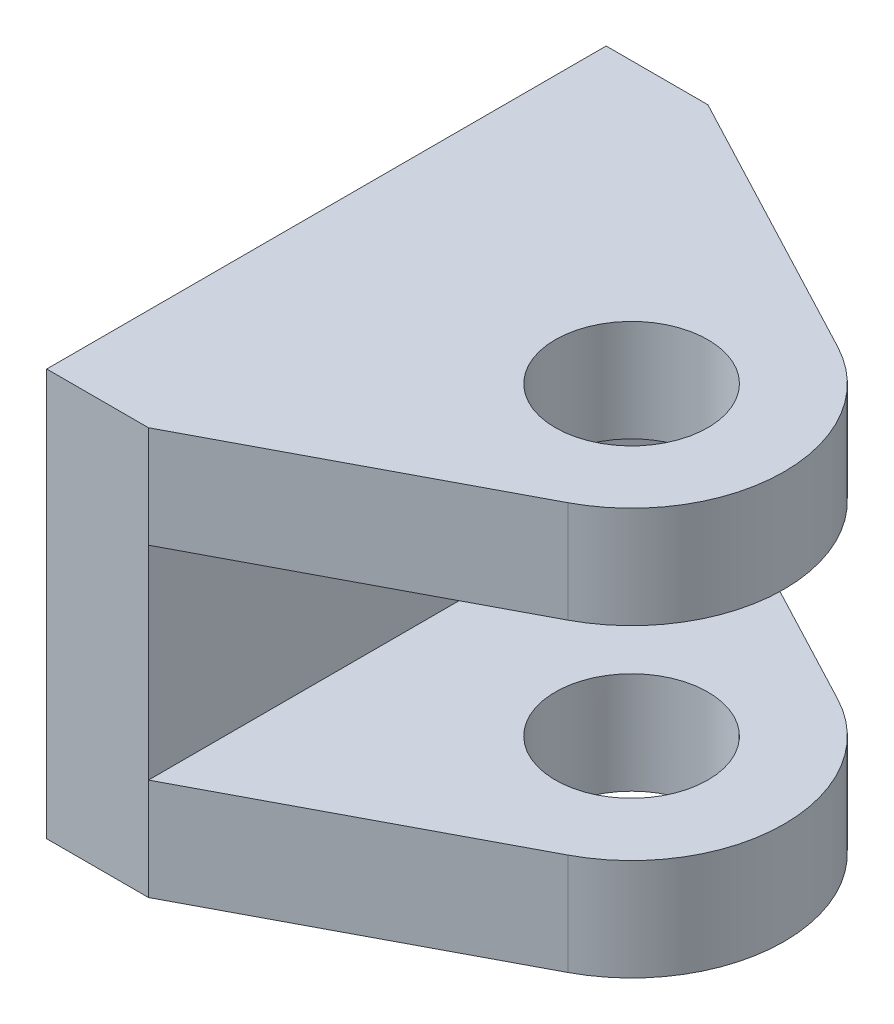
SolidWorks part; units mm, degrees
material "合金钢"
ref_plane "前视基准面" through (0, 0, 0) normal (0, 0, 1) x (1, 0, 0)
ref_plane "上视基准面" through (0, 0, 0) normal (0, 1, 0) x (1, 0, 0)
ref_plane "右视基准面" through (0, 0, 0) normal (1, 0, 0) x (0, 0, -1)
sketch "草图1" plane through (0, 0, 0) normal (0, 1, 0) x (1, 0, 0)
  line L0 (0, -27.5) -> (0, 27.5)
  line L1 (0, -27.5) -> (10, -27.5)
  line L2 (10, -27.5) -> (36.995, -13.2691)
  line L3 (0, 27.5) -> (10, 27.5)
  line L4 (10, 27.5) -> (36.995, 13.2691)
  arc A0 (36.995, -13.2691) -> (36.995, 13.2691) centre (30, 0) ccw
  circle A1 centre (30, 0) radius 7.5
  point P4 (0, 0)
  dimension "D1" = 30
  dimension "D2" = 15
  dimension "D3" = 10
  dimension "D4" = 10
  dimension "D5" = 30
  dimension "D6" = 55
extrude "凸台-拉伸1" add sketch "草图1" along normal blind 40
sketch "草图2" plane through (0, 0, -27.5) normal (0, 0, -1) x (-1, 0, 0)
  line L0 (-10, 40) -> (-10, 0) construction
  line L1 (-10, 30) -> (-64.9508, 30)
  line L2 (-10, 30) -> (-10, 10)
  line L3 (-10, 10) -> (-64.9508, 10)
  line L4 (-64.9508, 30) -> (-64.9508, 10)
  line L5 (-36.995, 0) -> (-10, 0) construction
  line L6 (-36.995, 40) -> (-10, 40) construction
  dimension "D1" = 10
  dimension "D2" = 10
extrude "切除-拉伸1" cut sketch "草图2" against normal through all
hole_wizard "M6 螺纹孔1" positions "草图3" profile "草图4" tap size "M6" standard "GB"
sketch "草图3" plane through (0, 0, 0) normal (-1, 0, 0) x (0, 0, 1)
  line L0 (-27.5, 40) -> (27.5, 40) construction
  line L1 (-27.5, 0) -> (27.5, 0) construction
  line L2 (-27.5, 40) -> (-27.5, 0) construction
  line L3 (27.5, 40) -> (27.5, 0) construction
  point P0 (-19.5, 5)
  point P2 (-19.5, 35)
  point P4 (19.5, 5)
  point P6 (19.5, 35)
  dimension "D1" = 5
  dimension "D2" = 5
  dimension "D3" = 8
  dimension "D4" = 8
sketch "草图4" plane through (0, 5, -19.5) normal (0, 1, 0) x (0, 0, 1)
  line L0 (0, 0) -> (0, 16.5022)
  line L1 (0, 16.5022) -> (2.5, 15)
  line L2 (2.5, 15) -> (2.5, 0)
  line L5 (2.5, 0) -> (0, 0)
  line L10 (0, 16.5022) -> (-2.5, 15) construction
  line L11 (0, -6.35) -> (0, 107.95) construction
  dimension "螺纹孔钻头直径" = 5
  dimension "螺纹孔钻头深度" = 15
  dimension "导头角度" = 118
cosmetic thread "孔螺蚊线1" parameters "D1"=12, "D2"=6
cosmetic thread "孔螺蚊线2" parameters "D1"=12, "D2"=6
cosmetic thread "孔螺蚊线3" parameters "D1"=12, "D2"=6
cosmetic thread "孔螺蚊线4" parameters "D1"=12, "D2"=6
chamfer "倒角1" [suppressed] distance 0.5 angle 45
